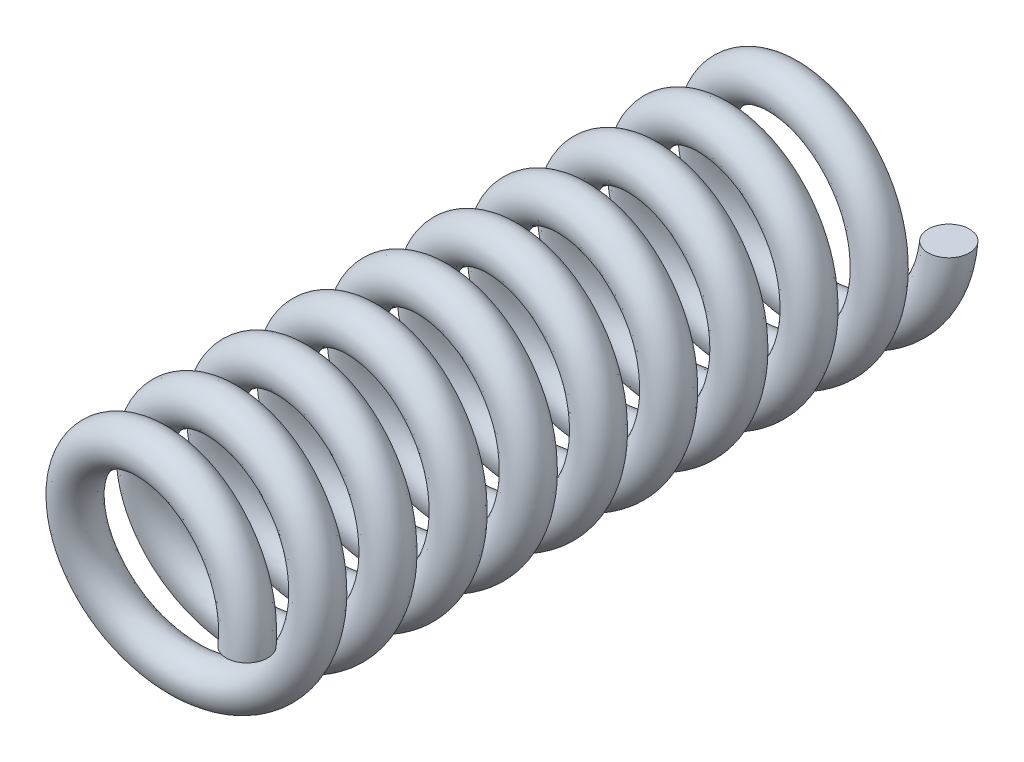
SolidWorks part; units mm, degrees
material "45"
ref_plane "前视基准面" through (0, 0, 0) normal (0, 0, 1) x (1, 0, 0)
ref_plane "上视基准面" through (0, 0, 0) normal (0, 1, 0) x (1, 0, 0)
ref_plane "右视基准面" through (0, 0, 0) normal (1, 0, 0) x (0, 0, -1)
sketch "草图1" plane through (0, 0, 0) normal (0, 0, 1) x (1, 0, 0)
  circle A0 centre (0, 0) radius 2.5
curve "螺旋线/涡状线1" pitch 1.7 height 17 turns 10
sketch "草图2" plane through (0, 0, 0) normal (0, 1, 0) x (1, 0, 0)
  circle A0 centre (2.5, 0) radius 0.5
sweep "扫描1" add profiles "草图2" path "螺旋线/涡状线1"
sketch "草图3" plane through (0, 0, 0) normal (0, 1, 0) x (1, 0, 0)
  line L0 (0, 0) -> (0, -20.5335)
